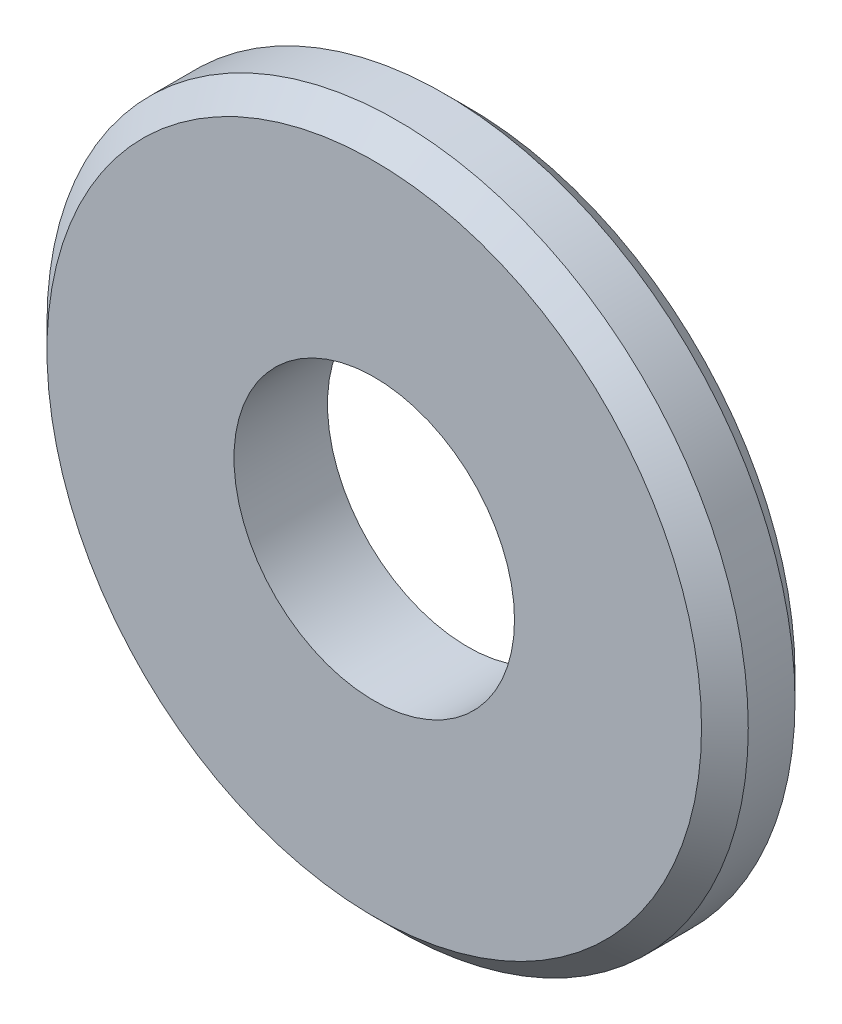
from build123d import *

# Parameters (mm, degrees)
SKETCH1_R           = 7.5
SKETCH1_R_2         = 3
BOSS_EXTRUDE1_DEPTH = 2
CHAMFER1_SIZE       = 0.5


with BuildPart() as part:
    # Sketch1 → Boss-Extrude1 (new body)
    with BuildSketch(Plane.XY):
        Circle(SKETCH1_R)
        Circle(SKETCH1_R_2, mode=Mode.SUBTRACT)
    extrude(amount=BOSS_EXTRUDE1_DEPTH)

    # Chamfer1
    chamfer1_edges = [part.edges().sort_by_distance(p)[0] for p in [
        (-7.5, 0, 0),
        (-7.5, 0, 2),
    ]]
    chamfer(chamfer1_edges, length=CHAMFER1_SIZE)


solid = part.part
